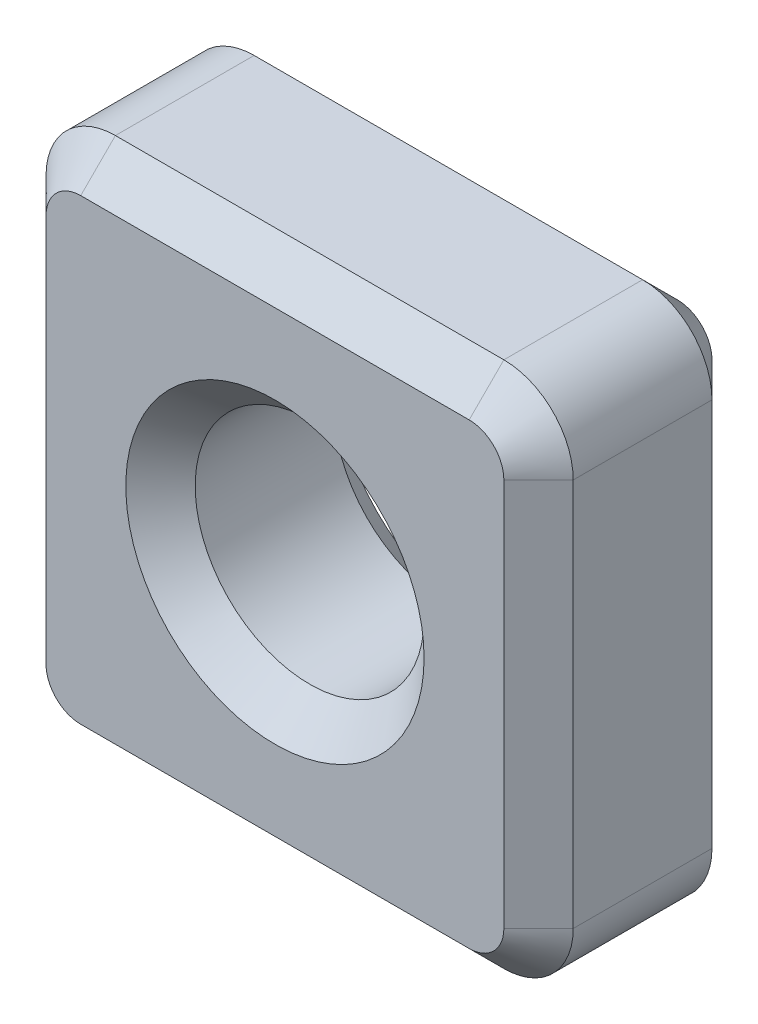
SolidWorks part; units mm, degrees
ref_plane "Front Plane" through (0, 0, 0) normal (0, 0, 1) x (1, 0, 0)
ref_plane "Top Plane" through (0, 0, 0) normal (0, 1, 0) x (1, 0, 0)
ref_plane "Right Plane" through (0, 0, 0) normal (1, 0, 0) x (0, 0, -1)
sketch "Sketch1" plane through (0, 0, 0) normal (0, 0, 1) x (1, 0, 0)
  line L1 (-2.8, 3.8) -> (2.8, 3.8)
  line L2 (-3.8, 2.8) -> (-3.8, -2.8)
  line L3 (-2.8, -3.8) -> (2.8, -3.8)
  line L4 (3.8, 2.8) -> (3.8, -2.8)
  line L5 (-3.8, 3.8) -> (3.8, -3.8) construction
  line L6 (-3.8, -3.8) -> (3.8, 3.8) construction
  arc A0 (-3.8, -2.8) -> (-2.8, -3.8) centre (-2.8, -2.8) ccw
  arc A1 (2.8, -3.8) -> (3.8, -2.8) centre (2.8, -2.8) ccw
  arc A2 (2.8, 3.8) -> (3.8, 2.8) centre (2.8, 2.8) cw
  arc A3 (-2.8, 3.8) -> (-3.8, 2.8) centre (-2.8, 2.8) ccw
  circle A4 centre (0, 0) radius 1.5
  point P0 (0, 0)
  dimension "D3" = 1
  dimension "D4" = 3
  dimension "D1" = 7.6
  dimension "D2" = 7.6
extrude "Boss-Extrude1" add sketch "Sketch1" along normal blind 3
hole_wizard "M4 Tapped Hole1" positions "Sketch3" profile "Sketch2" tap size "M4" standard "Iso"
sketch "Sketch3" plane through (0, 0, 0) normal (0, 0, -1) x (-1, 0, 0)
  point P0 (0, 0)
sketch "Sketch2" plane through (0, 0, 0) normal (1, 0, 0) x (0, 1, 0)
  line L0 (0, 0) -> (0, 12.4914)
  line L1 (0, 12.4914) -> (1.65, 11.5)
  line L2 (1.65, 11.5) -> (1.65, 0)
  line L5 (1.65, 0) -> (0, 0)
  line L10 (0, 12.4914) -> (-1.65, 11.5) construction
  line L11 (0, -6.35) -> (0, 107.95) construction
  dimension "螺纹孔钻头直径" = 3.3
  dimension "螺纹孔钻头深度" = 11.5
  dimension "导头角度" = 118
cosmetic thread "Cosmetic Thread1" parameters "D1"=3, "D2"=4
chamfer "Chamfer1" distance 0.5 angle 45 1 edges at (-1.65, 0, 0)
chamfer "Chamfer2" distance 0.5 angle 45 1 edges at (1.65, 0, 3)
chamfer "Chamfer3" distance 0.5 angle 45 16 edges at (-3.5071, 3.5071, 3) (-3.8, 0, 3) (-3.5071, -3.5071, 3) (0, -3.8, 3) (3.5071, -3.5071, 3) (3.8, 0, 3) (0, 3.8, 3) (3.5071, 3.5071, 3) (3.5071, -3.5071, 0) (3.8, 0, 0) (3.5071, 3.5071, 0) (0, 3.8, 0) (-3.5071, 3.5071, 0) (0, -3.8, 0) (-3.5071, -3.5071, 0) (-3.8, 0, 0)
